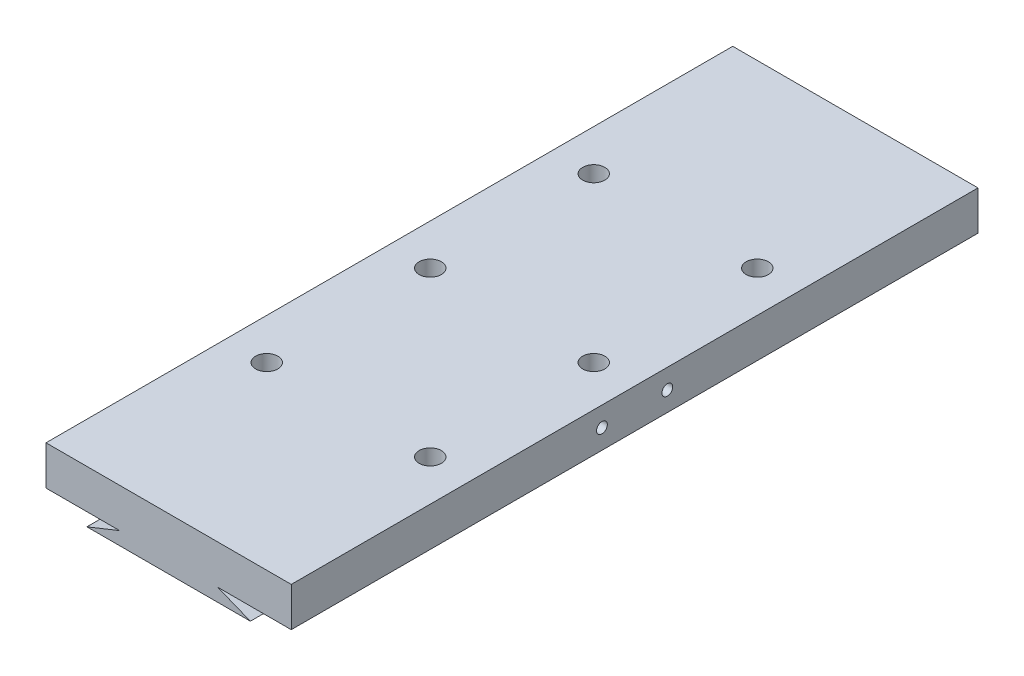
from build123d import *

# Parameters (mm, degrees)
EXTRUDE_1_DEPTH             = 105
HOLE_WIZARD_M4_1_AT_2_COUNT = 2
HOLE_WIZARD_M4_1_AT_2_PITCH = 20
PATTERN_LINEAR_1_COUNT      = 3
PATTERN_LINEAR_1_PITCH      = 50
PATTERN_LINEAR_1_COUNT_DIR2 = 2
PATTERN_LINEAR_1_PITCH_DIR2 = 50


with BuildPart() as part:
    # 草图1 → 凸台-拉伸1 (new, symmetric)
    with BuildSketch(Plane.XY):
        Polygon((-25, -10), (25, -10), (15, -6), (37.5, -6), (37.5, 6), (-37.5, 6), (-37.5, -6), (-15, -6), align=None)
    extrude(amount=EXTRUDE_1_DEPTH, both=True)

    # 草图2 → M4 螺纹孔1 (revolve, cut)
    with BuildSketch(Plane(origin=(-37.5, 0, -10), x_dir=(0, 0, 1), z_dir=(0, 1, 0))):
        Polygon((0, 0), (0, 11.091420021), (1.65, 10.1), (1.65, 0), align=None)
    hole_wizard_m4_1 = revolve(axis=Axis((-43.85, 0, -10), (1, 0, 0)), mode=Mode.SUBTRACT)

    # M4 螺纹孔1 at 2: M4 螺纹孔1 ×2
    with Locations(*[(0, 0, i * HOLE_WIZARD_M4_1_AT_2_PITCH) for i in range(1, HOLE_WIZARD_M4_1_AT_2_COUNT)]):
        add(hole_wizard_m4_1, mode=Mode.SUBTRACT)

    # 镜向1: M4 螺纹孔1 across plane
    add(hole_wizard_m4_1.mirror(Plane(origin=(0, 0, 0), x_dir=(0, 0, 1), z_dir=(1, 0, 0))), mode=Mode.SUBTRACT)

    # 镜向1 copy 1 sketch → 镜向1 copy 1 (revolve, cut)
    with BuildSketch(Plane(origin=(37.5, 0, 10), x_dir=(0, 0, 1), z_dir=(0, 1, 0))):
        Polygon((0, 0), (0, -11.091420021), (1.65, -10.1), (1.65, 0), align=None)
    revolve(axis=Axis((43.85, 0, 10), (1, 0, 0)), mode=Mode.SUBTRACT)

    # 草图4 → M8 螺纹孔1 (revolve, cut)
    with BuildSketch(Plane(origin=(-25, 6, -50), x_dir=(0, 0, 1), z_dir=(1, 0, 0))):
        Polygon((0, 0), (0, 21.792926105), (3.4, 19.75), (3.4, 0), align=None)
    hole_wizard_m8_1 = revolve(axis=Axis((-25, 12.35, -50), (0, -1, 0)), mode=Mode.SUBTRACT)

    # 阵列(线性)1: Hole Wizard M8 _1 3 × 2
    with Locations(*[(j * PATTERN_LINEAR_1_PITCH_DIR2, 0, i * PATTERN_LINEAR_1_PITCH) for i in range(PATTERN_LINEAR_1_COUNT) for j in range(PATTERN_LINEAR_1_COUNT_DIR2) if (i, j) != (0, 0)]):
        add(hole_wizard_m8_1, mode=Mode.SUBTRACT)


solid = part.part
